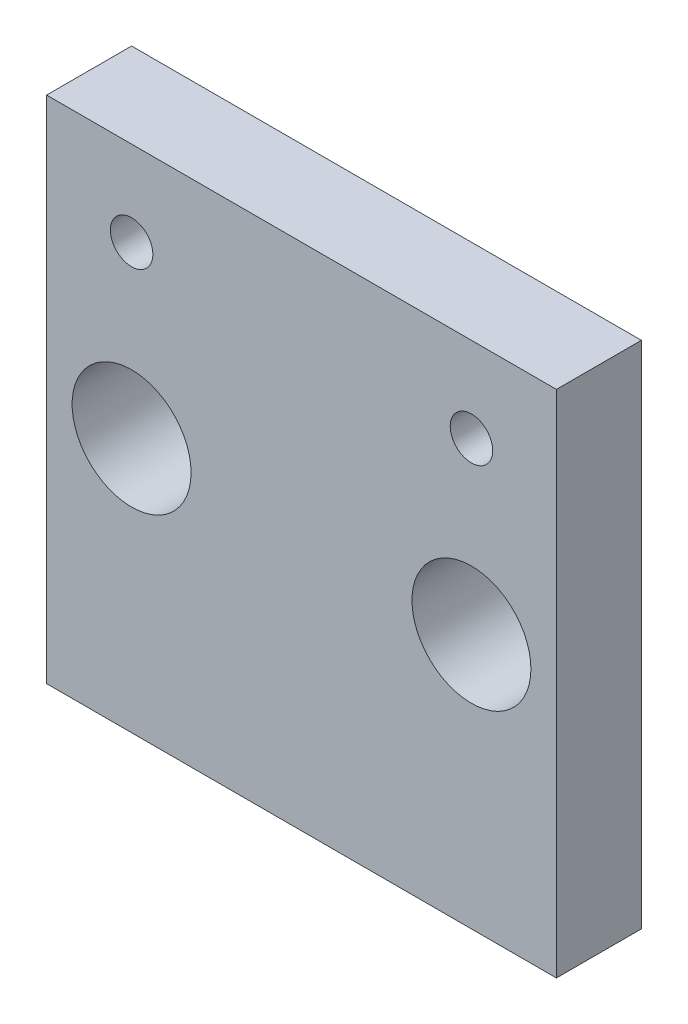
from build123d import *

# Parameters (mm, degrees)
SKETCH_1_W            = 30
SKETCH_1_H            = 30
SKETCH_1_R            = 1.25
EXTRUDE_1_DEPTH       = 5
HOLE_WIZARD_7_0_7_1_D = 7


with BuildPart() as part:
    # 草图1 → 凸台-拉伸1 (new body)
    with BuildSketch(Plane.XY.offset(5)):
        Rectangle(SKETCH_1_W, SKETCH_1_H)
        with Locations(Location((-10, 10, 0), (0, 0, 180))):
            Circle(SKETCH_1_R, mode=Mode.SUBTRACT)
        with Locations(Location((10, 10, 0), (0, 0, 180))):
            Circle(SKETCH_1_R, mode=Mode.SUBTRACT)
    extrude(amount=-EXTRUDE_1_DEPTH)

    # Ø7.0 (7) 直径孔1 (through all)
    with Locations(Plane.XY.offset(5)):
        with Locations((10, 0), (-10, 0)):
            Hole(HOLE_WIZARD_7_0_7_1_D / 2)


solid = part.part
